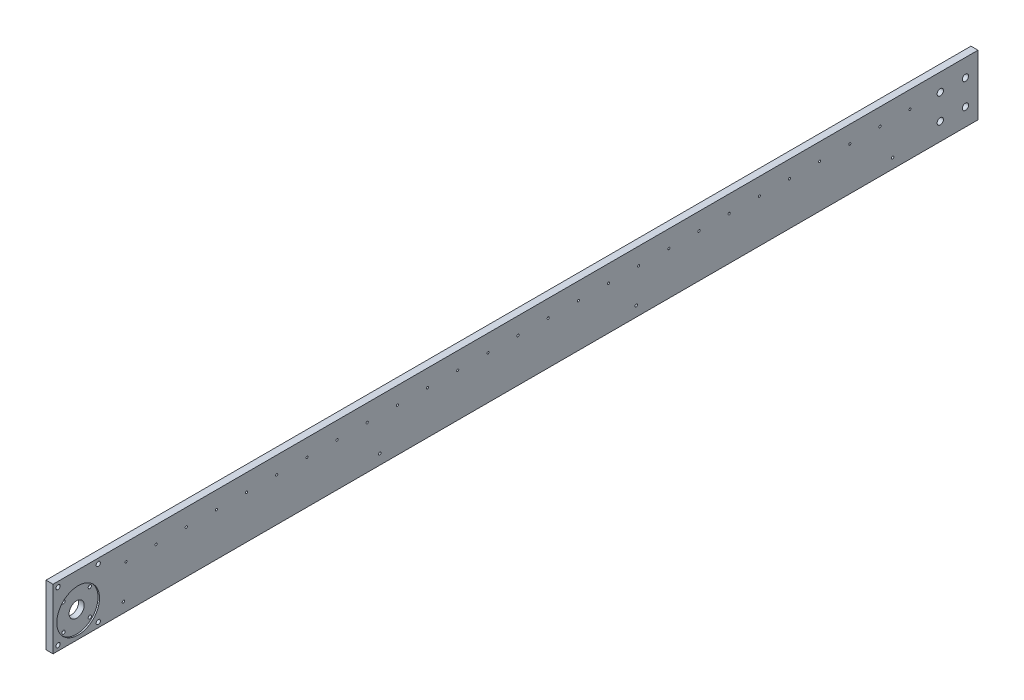
from build123d import *

# Parameters (mm, degrees)
SKETCH_1_W                = 1840
SKETCH_1_H                = 120
EXTRUDE_1_DEPTH           = 14
HOLE_WIZARD_1_D           = 6.6
HOLE_WIZARD_1_CBORE_D     = 11
HOLE_WIZARD_1_CBORE_DEPTH = 6.8
HOLE_WIZARD_M5_1_D        = 4.2
PATTERN_LINEAR_1_COUNT    = 27
PATTERN_LINEAR_1_PITCH    = 60
HOLE_WIZARD_12_5_12_5_2_D = 12.5
SKETCH_8_R                = 15
CUT_EXTRUDE_1_DEPTH       = 923.060735527
HOLE_WIZARD_M6_1_D        = 5
PATTERN_LINEAR_2_COUNT    = 4
PATTERN_LINEAR_2_PITCH    = 510
HOLE_WIZARD_8_5_8_5_1_D   = 8.5
SKETCH_13_R               = 42.5
CUT_EXTRUDE_2_DEPTH       = 3


with BuildPart() as part:
    # 草图1 → 凸台-拉伸1 (new body)
    with BuildSketch(Plane(origin=(0, 0, 0), x_dir=(0, 0, -1), z_dir=(1, 0, 0))):
        Rectangle(SKETCH_1_W, SKETCH_1_H)
    extrude(amount=EXTRUDE_1_DEPTH)

    # 打孔尺寸(%根据)内六角圆柱头螺钉的类型1 (through all)
    with Locations(Plane(origin=(0, 0, 0), x_dir=(0, 0, -1), z_dir=(-1, 0, 0))):
        with Locations((-896.162950904, -16.162950904), (-843.837049096, -16.162950904), (-896.162950904, 36.162950904), (-843.837049096, 36.162950904)):
            CounterBoreHole(HOLE_WIZARD_1_D / 2, HOLE_WIZARD_1_CBORE_D / 2, HOLE_WIZARD_1_CBORE_DEPTH)

    # M5 螺纹孔1 (through all)
    with Locations(Plane(origin=(14, 0, 0), x_dir=(0, 0, -1), z_dir=(1, 0, 0))):
        with Locations((-775, 26)):
            hole_wizard_m5_1 = Hole(HOLE_WIZARD_M5_1_D / 2)

    # 阵列(线性)1: M5 螺纹孔1 ×27
    with Locations(*[(0, 0, -i * PATTERN_LINEAR_1_PITCH) for i in range(1, PATTERN_LINEAR_1_COUNT)]):
        add(hole_wizard_m5_1, mode=Mode.SUBTRACT)

    # Ø12.5 (12.5) 直径孔2 (through all)
    with Locations(Plane(origin=(14, 0, 0), x_dir=(0, 0, -1), z_dir=(1, 0, 0))):
        with Locations((845, 25), (895, 25), (845, -25), (895, -25)):
            Hole(HOLE_WIZARD_12_5_12_5_2_D / 2)

    # 草图8 → 切除-拉伸1 (cut, through all)
    with BuildSketch(Plane(origin=(14, 0, 0), x_dir=(0, 0, -1), z_dir=(1, 0, 0))):
        with Locations((-870, -10)):
            Circle(SKETCH_8_R)
    extrude(amount=-CUT_EXTRUDE_1_DEPTH, mode=Mode.SUBTRACT)

    # M6 螺纹孔1 (through all)
    with Locations(Plane.ZY):
        with Locations((780, -40)):
            hole_wizard_m6_1 = Hole(HOLE_WIZARD_M6_1_D / 2)

    # 阵列(线性)2: M6 螺纹孔1 ×4
    with Locations(*[(0, 0, -i * PATTERN_LINEAR_2_PITCH) for i in range(1, PATTERN_LINEAR_2_COUNT)]):
        add(hole_wizard_m6_1, mode=Mode.SUBTRACT)

    # Ø8.5 (8.5) 直径孔1 (through all)
    with Locations(Plane(origin=(14, 0, 0), x_dir=(0, 0, -1), z_dir=(1, 0, 0))):
        with Locations((-910, 50), (-830, 50), (-910, -50), (-830, -50)):
            Hole(HOLE_WIZARD_8_5_8_5_1_D / 2)

    # 草图13 → 切除-拉伸2 (cut)
    with BuildSketch(Plane(origin=(14, 0, 0), x_dir=(0, 0, -1), z_dir=(1, 0, 0))):
        with Locations((-870, -10)):
            Circle(SKETCH_13_R)
    extrude(amount=-CUT_EXTRUDE_2_DEPTH, mode=Mode.SUBTRACT)


solid = part.part
